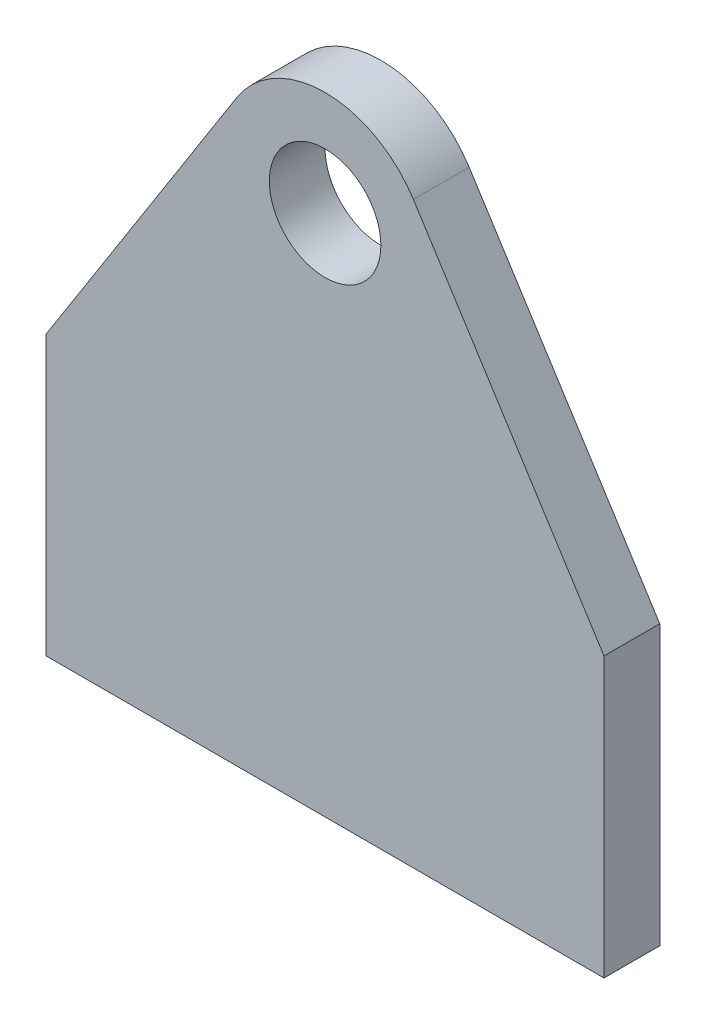
SolidWorks part; units mm, degrees
material "Q235"
ref_plane "Front Plane" through (0, 0, 0) normal (0, 0, 1) x (1, 0, 0)
ref_plane "Top Plane" through (0, 0, 0) normal (0, 1, 0) x (1, 0, 0)
ref_plane "Right Plane" through (0, 0, 0) normal (1, 0, 0) x (0, 0, -1)
sketch "Sketch1" plane through (0, 0, 0) normal (0, 0, 1) x (1, 0, 0)
  line L0 (0, 0) -> (0, 40)
  line L1 (0, 0) -> (80, 0)
  line L2 (80, 0) -> (80, 40)
  line L3 (80, 40) -> (52.6619, 83.0422)
  line L4 (0, 40) -> (27.3381, 83.0422)
  line L5 (40, 75) -> (40, 0) construction
  arc A0 (52.6619, 83.0422) -> (27.3381, 83.0422) centre (40, 75) ccw
  circle A1 centre (40, 75) radius 8
  dimension "D4" = 30
  dimension "D5" = 16
  dimension "D1" = 40
  dimension "D2" = 75
  dimension "D3" = 80
extrude "Boss-Extrude1" add sketch "Sketch1" along normal blind 8
